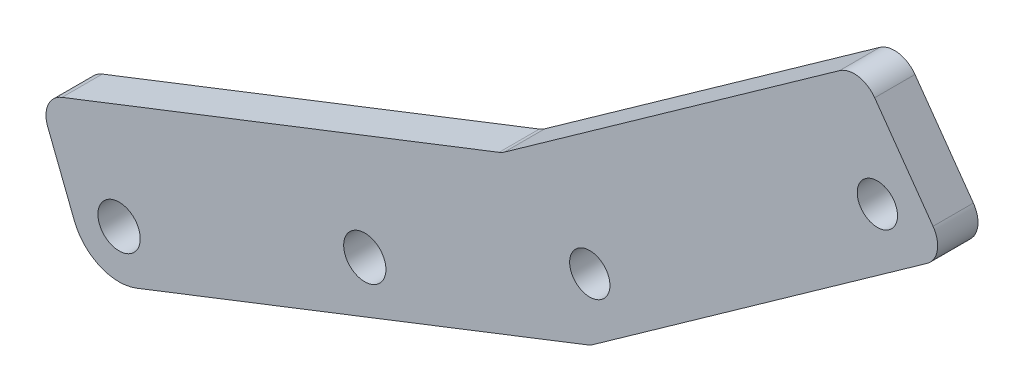
SolidWorks part; units mm, degrees
ref_plane "前视基准面" through (0, 0, 0) normal (0, 0, 1) x (1, 0, 0)
ref_plane "上视基准面" through (0, 0, 0) normal (0, 1, 0) x (1, 0, 0)
ref_plane "右视基准面" through (0, 0, 0) normal (1, 0, 0) x (0, 0, -1)
sketch "草图1" plane through (0, 0, 0) normal (0, 0, 1) x (1, 0, 0)
  line L1 (87.9794, 127.6107) -> (-1.5294, 92.6062)
  line L2 (155.3727, 175.3133) -> (89.0544, 128.1914)
  line L4 (158.3653, 65.7866) -> (212.1682, 104.013)
  line L5 (-13.8693, 98.0078) -> (-19.1595, 111.5352)
  line L6 (156.5525, 182.2852) -> (144.9682, 198.5887)
  line L7 (11.7543, 97.8011) -> (11.5783, 97.676)
  line L9 (137.9962, 199.7685) -> (71.4955, 152.517)
  line L11 (70.4205, 151.9363) -> (-16.324, 118.0128)
  circle A0 centre (43.7683, 120.5484) radius 4.191
  circle A1 centre (-4.9986, 101.477) radius 4.2
  arc A2 (-13.8693, 98.0078) -> (-1.5294, 92.6062) centre (-4.9986, 101.477) ccw
  arc A3 (156.5525, 182.2852) -> (155.3727, 175.3133) centre (152.4766, 179.3891) cw
  circle A4 centre (158.3653, 65.7866) radius 66 construction
  circle A5 centre (158.3653, 65.7866) radius 66
  arc A6 (144.9682, 198.5887) -> (137.9962, 199.7685) centre (140.8923, 195.6926) ccw
  arc A7 (-16.324, 118.0128) -> (-19.1595, 111.5352) centre (-14.5029, 113.3563) ccw
  arc A8 (87.9794, 127.6107) -> (89.0544, 128.1914) centre (86.1583, 132.2672) ccw
  arc A9 (71.4955, 152.517) -> (70.4205, 151.9363) centre (68.5994, 156.5929) cw
  point P10 (153.1167, 198.2449)
  point P12 (164.701, 181.9414)
  point P13 (23.1626, 81.3725)
  point P19 (143.7884, 191.6168)
  point P27 (76.2841, 143.6522)
  dimension "D1" = 20
  dimension "D2" = 5
extrude "凸台-拉伸1" add sketch "草图1" along normal blind 8
sketch "草图2" plane through (0, 0, 8) normal (0, 0, 1) x (1, 0, 0)
  line L0 (88.5347, 127.868) -> (99.7805, 135.8509) construction
  line L1 (155.3727, 175.3133) -> (89.0544, 128.1914) construction
  line L2 (156.5525, 182.2852) -> (144.9682, 198.5887) construction
  arc A0 (87.9794, 127.6107) -> (89.0544, 128.1914) centre (86.1583, 132.2672) ccw construction
  circle A1 centre (145.5047, 180.5689) radius 4
  circle A2 centre (88.4226, 140.0518) radius 4
  point P1 (82.7462, 136.0224)
  point P6 (164.869, 194.3176)
  point P8 (170.6575, 186.1632)
  dimension "D1" = 8
  dimension "D2" = 8
  dimension "D6" = 70
  dimension "D3" = 10
  dimension "D4" = 10
  dimension "D5" = 10
extrude "切除-拉伸1" cut sketch "草图2" against normal blind 20
